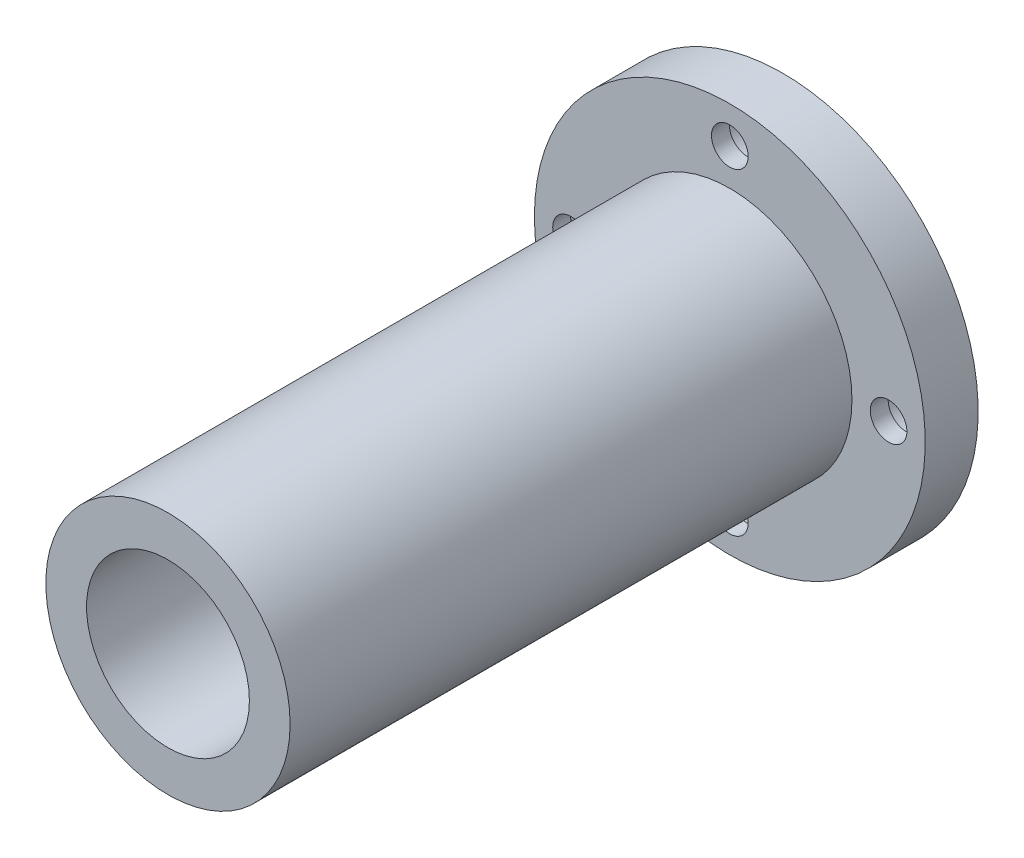
SolidWorks part; units mm, degrees
ref_plane "前视基准面" through (0, 0, 0) normal (0, 0, 1) x (1, 0, 0)
ref_plane "上视基准面" through (0, 0, 0) normal (0, 1, 0) x (1, 0, 0)
ref_plane "右视基准面" through (0, 0, 0) normal (1, 0, 0) x (0, 0, -1)
sketch "草图1" plane through (0, 0, 0) normal (0, 0, 1) x (1, 0, 0)
  circle A0 centre (0, 0) radius 48
  dimension "D1" = 96
extrude "拉伸1" add sketch "草图1" along normal blind 13
hole_wizard "M8 六角凹头螺钉的柱形沉头孔1" positions "3D草图1" profile "草图2" counterbore size "M8" standard "ISO" end condition through all
sketch3d "3D草图1"
  line L0 (0, 39, 0) -> (0, -39, 0) construction
  line L3 (39, 0, 0) -> (-39, 0, 0) construction
  circle A0 centre (0, 0, 0) radius 39 construction
  point P0 (0, 39, 0)
  point P2 (39, 0, 0)
  point P4 (0, -39, 0)
  point P6 (-39, 0, 0)
  point P11 (0, 0, 39)
  dimension "D1" = 78
sketch "草图2" plane through (0, 39, 0) normal (1, 0, 0) x (0, 1, 0)
  line L0 (0, 0) -> (0, 13)
  line L1 (0, 13) -> (4.5, 13)
  line L3 (4.5, 13) -> (4.5, 8.6)
  line L4 (4.5, 8.6) -> (7, 8.6)
  line L5 (7, 8.6) -> (7, 0)
  line L7 (7, 0) -> (0, 0)
  line L11 (0, -6.35) -> (0, 107.95) construction
  dimension "通孔孔直径" = 9
  dimension "通孔孔深度" = 13
  dimension "柱形沉头孔直径" = 14
  dimension "柱形沉头孔深度" = 8.6
sketch "草图3" plane through (0, 0, 13) normal (0, 0, 1) x (1, 0, 0)
  circle A0 centre (0, 0) radius 30
  dimension "D1" = 60
extrude "拉伸2" add sketch "草图3" along normal blind 138
sketch "草图4" plane through (0, 0, 151) normal (0, 0, 1) x (1, 0, 0)
  circle A0 centre (0, 0) radius 20
  dimension "D1" = 40
extrude "拉伸3" cut sketch "草图4" against normal through all
